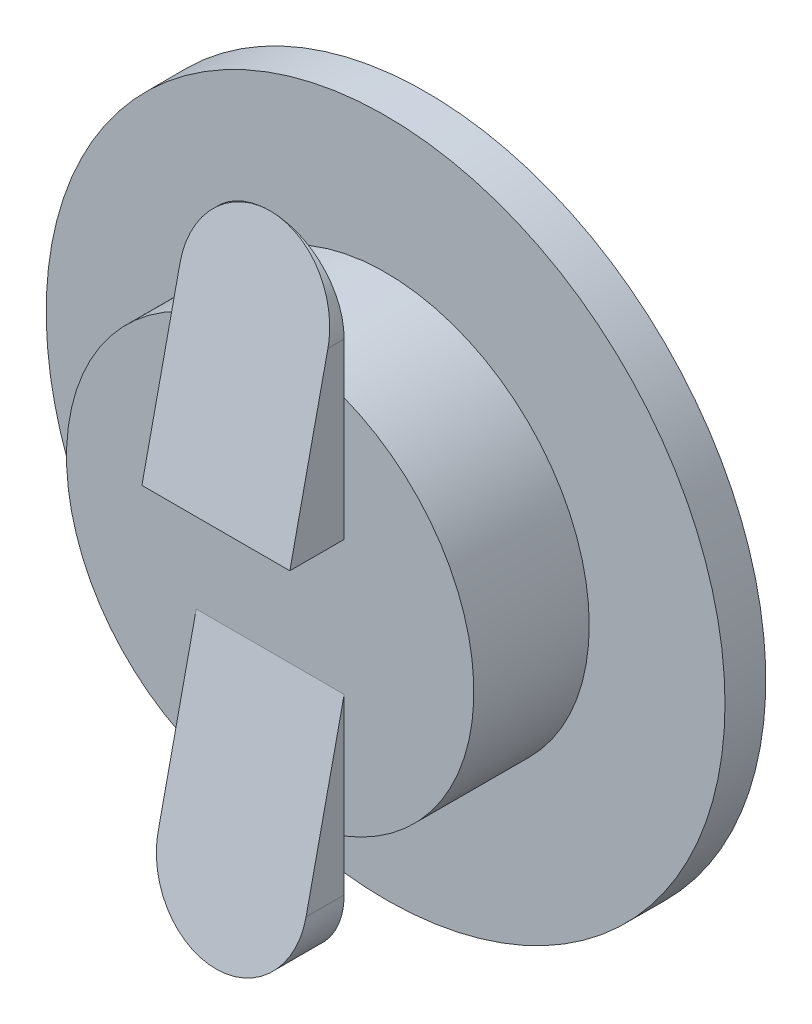
from build123d import *
from build123d.topology import SkipClean

# Parameters (mm, degrees)
SKETCH1_R           = 25
BOSS_EXTRUDE1_DEPTH = 1.5
BOSS_EXTRUDE2_DEPTH = 8
CUT_EXTRUDE2_DEPTH  = 8
SKETCH4_R           = 15
BOSS_EXTRUDE3_DEPTH = 8.5
BOSS_EXTRUDE4_DEPTH = 4
CUT_EXTRUDE3_DEPTH  = 42.809799474


with BuildPart() as part:
    # Sketch1 → Boss-Extrude1 (new, symmetric)
    with BuildSketch(Plane.XY):
        Circle(SKETCH1_R)
    extrude(amount=BOSS_EXTRUDE1_DEPTH, both=True)

    # Sketch2 → Boss-Extrude2 (add)
    with SkipClean():  # the faces are left unmerged after this step: merging them gives an invalid solid
        with BuildSketch(Plane(origin=(0, 0, -1.5), x_dir=(-1, 0, 0), z_dir=(0, 0, -1))):
            with BuildLine():
                Line((24.840821943, 2.816658516), (-24.840821943, 2.816658516))
                ThreePointArc((-24.840821943, 2.816658516), (-25, 0), (-24.840821943, -2.816658516))
                Line((-24.840821943, -2.816658516), (24.840821943, -2.816658516))
                ThreePointArc((24.840821943, -2.816658516), (24.960173763, -1.410576376), (25, 0))
                ThreePointArc((25, 0), (24.960173763, 1.410576376), (24.840821943, 2.816658516))
            make_face()
        extrude(amount=BOSS_EXTRUDE2_DEPTH)

    # Sketch3 → Cut-Extrude2 (cut)
    with BuildSketch(Plane(origin=(0, 2.816658516, 0), x_dir=(1, 0, 0), z_dir=(0, 1, 0))):
        Polygon((-29.660487574, 11.299873817), (-29.660487574, 1.5), (-24.840821943, 1.5), (-24.840821943, 9.5), (24.840821943, 9.5), (24.840821943, 1.5), (29.900960726, 1.5), (29.900960726, 11.299873817), align=None)
        with BuildLine():
            ThreePointArc((-24.840821943, 1.5), (0, 8.954423408), (24.840821943, 1.5))
            Line((24.840821943, 1.5), (24.840821943, 9.5))
            Line((24.840821943, 9.5), (-24.840821943, 9.5))
            Line((-24.840821943, 9.5), (-24.840821943, 1.5))
        make_face()
    extrude(amount=-CUT_EXTRUDE2_DEPTH, mode=Mode.SUBTRACT)

    # Sketch4 → Boss-Extrude3 (add)
    with BuildSketch(Plane.XY.offset(1.5)):
        Circle(SKETCH4_R)
    extrude(amount=BOSS_EXTRUDE3_DEPTH)

    # Sketch5 → Boss-Extrude4 (add)
    with BuildSketch(Plane.XY.offset(10)):
        with BuildLine():
            Line((-5.44764904, 17.730849129), (-5.44764904, 4.943959841))
            Line((-5.44764904, 4.943959841), (5.44764904, 4.943959841))
            Line((5.44764904, 4.943959841), (5.44764904, 17.730849129))
            ThreePointArc((5.44764904, 17.730849129), (0, 23.17849817), (-5.44764904, 17.730849129))
        make_face()
        with BuildLine():
            Line((-5.44764904, -17.730849129), (-5.44764904, -4.943959841))
            Line((-5.44764904, -4.943959841), (5.44764904, -4.943959841))
            Line((5.44764904, -4.943959841), (5.44764904, -17.730849129))
            ThreePointArc((5.44764904, -17.730849129), (0, -23.17849817), (-5.44764904, -17.730849129))
        make_face()
    extrude(amount=BOSS_EXTRUDE4_DEPTH)

    # Sketch7 → Cut-Extrude3 (cut, through all)
    with BuildSketch(Plane.ZY.offset(5.44764904)):
        Polygon((10, 23.17849817), (14, 4.943959841), (14, 23.17849817), align=None)
        Polygon((14, -23.17849817), (10, -4.943959841), (14, -4.943959841), align=None)
    extrude(amount=-CUT_EXTRUDE3_DEPTH, mode=Mode.SUBTRACT)


solid = part.part
